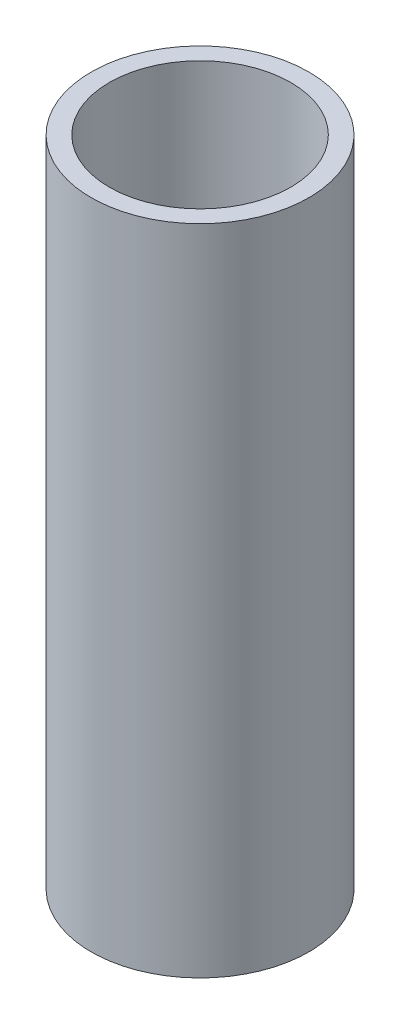
SolidWorks part; units mm, degrees
ref_plane "Front Plane" through (0, 0, 0) normal (0, 0, 1) x (1, 0, 0)
ref_plane "Top Plane" through (0, 0, 0) normal (0, 1, 0) x (1, 0, 0)
ref_plane "Right Plane" through (0, 0, 0) normal (1, 0, 0) x (0, 0, -1)
sketch "Sketch 1" plane through (0, 0, 0) normal (0, 1, 0) x (1, 0, 0)
  circle A0 centre (0, 0) radius 25
  circle A1 centre (0, 0) radius 30
  dimension "D1" = 60
  dimension "D2" = 50
extrude "Boss-Extrude 1" add sketch "Sketch 1" along normal mid plane 180
